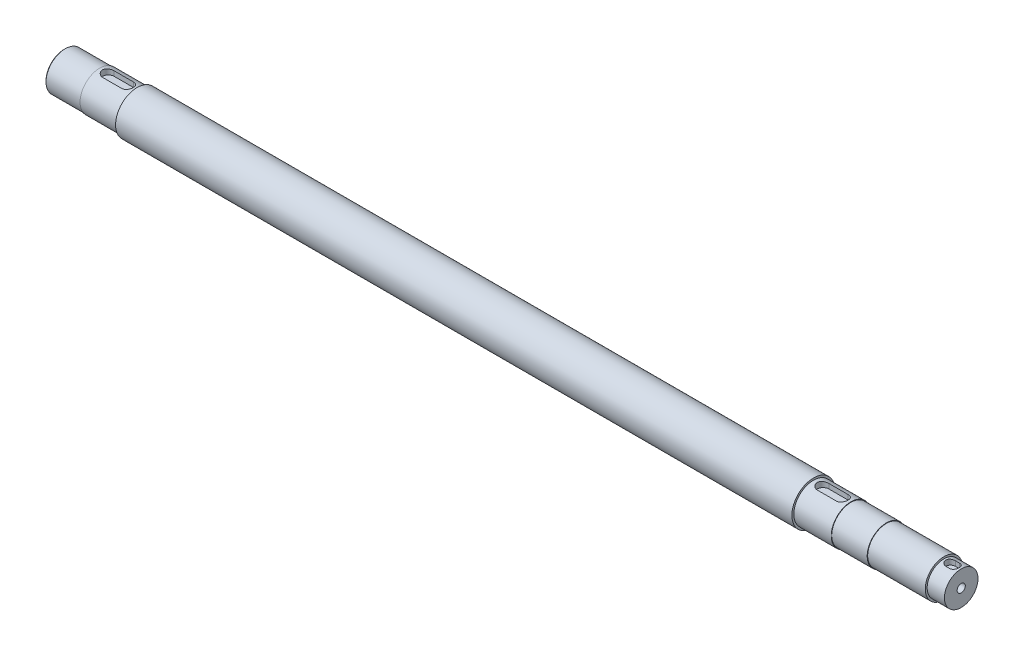
from build123d import *

# Parameters (mm, degrees)
SKETCH_1_R              = 22.5
EXTRUDE_1_DEPTH         = 705
SKETCH_2_R              = 20.5
EXTRUDE_2_DEPTH         = 39
SKETCH_3_R              = 20
EXTRUDE_3_DEPTH         = 37
SKETCH_4_R              = 19.5
EXTRUDE_4_DEPTH         = 60
SKETCH_5_R              = 17.5
EXTRUDE_5_DEPTH         = 18
EXTRUDE_START           = 39
SKETCH_6_R              = 20.5
EXTRUDE_6_DEPTH         = 39
EXTRUDE_START_2         = 37
SKETCH_7_R              = 20
EXTRUDE_7_DEPTH         = 37
CHAMFER_1_SIZE          = 1
CUT_EXTRUDE_1_DEPTH     = 5.9
CUT_EXTRUDE_2_DEPTH     = 5.73
HOLE_WIZARD_M10_1_D     = 8.5
HOLE_WIZARD_M10_1_DEPTH = 15
HOLE_WIZARD_M10_1_TIP   = 2.553657631


with BuildPart() as part:
    # 草图1 → 凸台-拉伸1 (new body)
    with BuildSketch(Plane(origin=(0, 0, 0), x_dir=(0, 0, -1), z_dir=(1, 0, 0))):
        Circle(SKETCH_1_R)
    extrude(amount=EXTRUDE_1_DEPTH)

    # 草图2 → 凸台-拉伸2 (add)
    with BuildSketch(Plane(origin=(705, 0, 0), x_dir=(0, 0, -1), z_dir=(1, 0, 0))):
        Circle(SKETCH_2_R)
    extrude(amount=EXTRUDE_2_DEPTH)

    # 草图3 → 凸台-拉伸3 (add)
    with BuildSketch(Plane(origin=(744, 0, 0), x_dir=(0, 0, -1), z_dir=(1, 0, 0))):
        Circle(SKETCH_3_R)
    extrude(amount=EXTRUDE_3_DEPTH)

    # 草图4 → 凸台-拉伸4 (add)
    with BuildSketch(Plane(origin=(781, 0, 0), x_dir=(0, 0, -1), z_dir=(1, 0, 0))):
        Circle(SKETCH_4_R)
    extrude(amount=EXTRUDE_4_DEPTH)

    # 草图5 → 凸台-拉伸5 (add)
    with BuildSketch(Plane(origin=(841, 0, 0), x_dir=(0, 0, -1), z_dir=(1, 0, 0))):
        Circle(SKETCH_5_R)
    extrude(amount=EXTRUDE_5_DEPTH)

    # 草图6 → 凸台-拉伸6 (add)
    with BuildSketch(Plane.ZY.offset(EXTRUDE_START)):
        with Locations(Location((0, 0, 0), (0, 0, 180))):
            Circle(SKETCH_6_R)
    extrude(amount=-EXTRUDE_6_DEPTH)

    # 草图7 → 凸台-拉伸7 (add)
    with BuildSketch(Plane.ZY.offset(39).offset(EXTRUDE_START_2)):
        with Locations(Location((0, 0, 0), (0, 0, 180))):
            Circle(SKETCH_7_R)
    extrude(amount=-EXTRUDE_7_DEPTH)

    # 倒角1
    chamfer_1_edges = [part.edges().sort_by_distance(p)[0] for p in [
        (-76, 0, 20),
    ]]
    chamfer(chamfer_1_edges, length=CHAMFER_1_SIZE)

    # 草图8 → 切除-拉伸1 (cut)
    with BuildSketch(Plane(origin=(0, 20.5, 0), x_dir=(1, 0, 0), z_dir=(0, 1, 0))):
        with BuildLine():
            Line((-10, -6), (-30, -6))
            ThreePointArc((-30, -6), (-36, 0), (-30, 6))
            Line((-30, 6), (-10, 6))
            ThreePointArc((-10, 6), (-4, 0), (-10, -6))
        make_face()
        with BuildLine():
            Line((715, 6), (735, 6))
            ThreePointArc((735, 6), (741, 0), (735, -6))
            Line((735, -6), (715, -6))
            ThreePointArc((715, -6), (709, 0), (715, 6))
        make_face()
    extrude(amount=-CUT_EXTRUDE_1_DEPTH, mode=Mode.SUBTRACT)

    # 草图9 → 切除-拉伸2 (cut)
    with BuildSketch(Plane(origin=(0, 17.5, 0), x_dir=(1, 0, 0), z_dir=(0, 1, 0))):
        with BuildLine():
            Line((848, 5), (852, 5))
            ThreePointArc((852, 5), (857, 0), (852, -5))
            Line((852, -5), (848, -5))
            ThreePointArc((848, -5), (843, 0), (848, 5))
        make_face()
    extrude(amount=-CUT_EXTRUDE_2_DEPTH, mode=Mode.SUBTRACT)

    # M10 螺纹孔1
    with Locations(Plane(origin=(859, 0, 0), x_dir=(0, 0, -1), z_dir=(1, 0, 0))):
        with Locations((0, 0)):
            Hole(HOLE_WIZARD_M10_1_D / 2, depth=HOLE_WIZARD_M10_1_DEPTH)
            with Locations((0, 0, -(HOLE_WIZARD_M10_1_DEPTH + HOLE_WIZARD_M10_1_TIP / 2))):  # 118° drill point
                Cone(0, HOLE_WIZARD_M10_1_D / 2, HOLE_WIZARD_M10_1_TIP, mode=Mode.SUBTRACT)


solid = part.part
